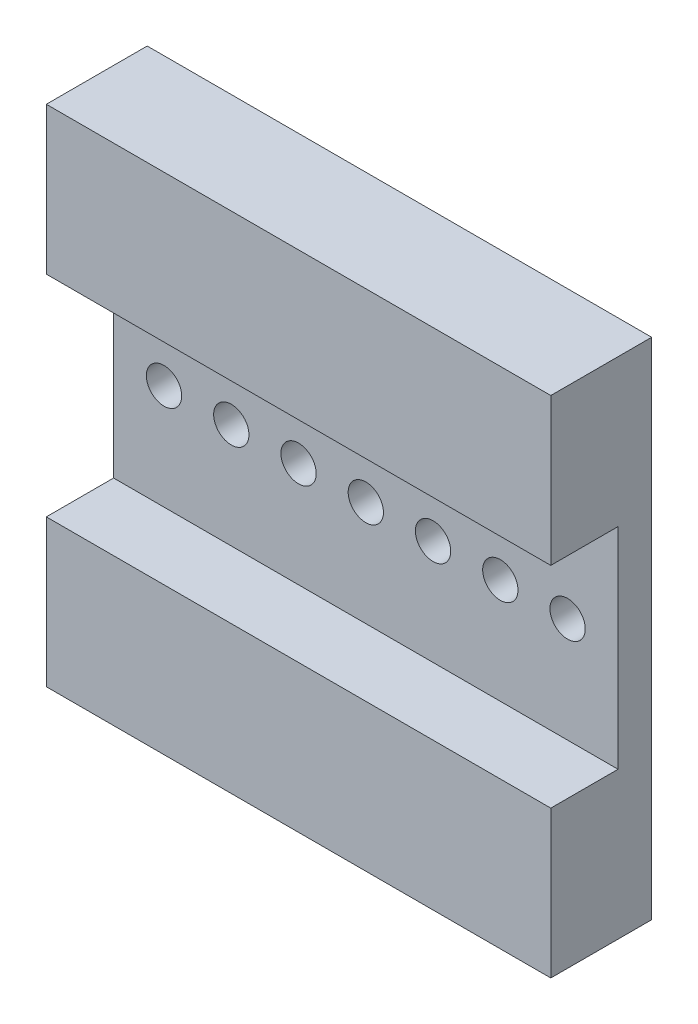
SolidWorks part; units mm, degrees
ref_plane "前视基准面" through (0, 0, 0) normal (0, 0, 1) x (1, 0, 0)
ref_plane "上视基准面" through (0, 0, 0) normal (0, 1, 0) x (1, 0, 0)
ref_plane "右视基准面" through (0, 0, 0) normal (1, 0, 0) x (0, 0, -1)
sketch "草图1" plane through (0, 0, 0) normal (0, 0, 1) x (1, 0, 0)
  line L1 (-30, -30) -> (30, -30)
  line L2 (-30, -30) -> (-30, 30)
  line L3 (-30, 30) -> (30, 30)
  line L4 (30, -30) -> (30, 30)
  line L5 (-30, -30) -> (30, 30) construction
  line L6 (-30, 30) -> (30, -30) construction
  point P0 (0, 0)
  dimension "D1" = 60
  dimension "D2" = 60
extrude "凸台-拉伸1" add sketch "草图1" along normal blind 12
sketch "草图2" plane through (0, 0, 12) normal (0, 0, 1) x (1, 0, 0)
  line L1 (-30, -12.5) -> (30, -12.5)
  line L2 (-30, -12.5) -> (-30, 12.5)
  line L3 (-30, 12.5) -> (30, 12.5)
  line L4 (30, -12.5) -> (30, 12.5)
  line L5 (-30, -12.5) -> (30, 12.5) construction
  line L6 (-30, 12.5) -> (30, -12.5) construction
  line L7 (30, -30) -> (30, 30) construction
  point P0 (0, 0)
  dimension "D1" = 25
extrude "切除-拉伸1" cut sketch "草图2" against normal blind 8
hole_wizard "M5 螺纹孔1" positions "3D草图2" profile "草图3" tap size "M5" standard "GB" end condition through all
sketch3d "3D草图2"
  line L0 (0, -12.5, 4) -> (0, 12.5, 4) construction
  line L1 (-30, -12.5, 4) -> (30, -12.5, 4) construction
  line L2 (30, 12.5, 4) -> (-30, 12.5, 4) construction
  point P0 (0, 0, 4)
sketch "草图3" plane through (0, 0, 4) normal (1, 0, 0) x (0, -1, 0)
  line L0 (0, 0) -> (0, 4)
  line L1 (0, 4) -> (2.1, 4)
  line L2 (2.1, 4) -> (2.1, 0)
  line L5 (2.1, 0) -> (0, 0)
  line L11 (0, -6.35) -> (0, 107.95) construction
  dimension "通孔螺纹孔钻头直径" = 4.2
  dimension "通孔螺纹孔钻头深度" = 4
cosmetic thread "孔螺蚊线1" parameters "D2"=5
pattern_linear "阵列(线性)1" count 4 spacing 8 along (-1, 0, 0) of "M5 螺纹孔1"
mirror "镜向1" about plane through (0, 0, 0) normal (1, 0, 0) of "阵列(线性)1"
